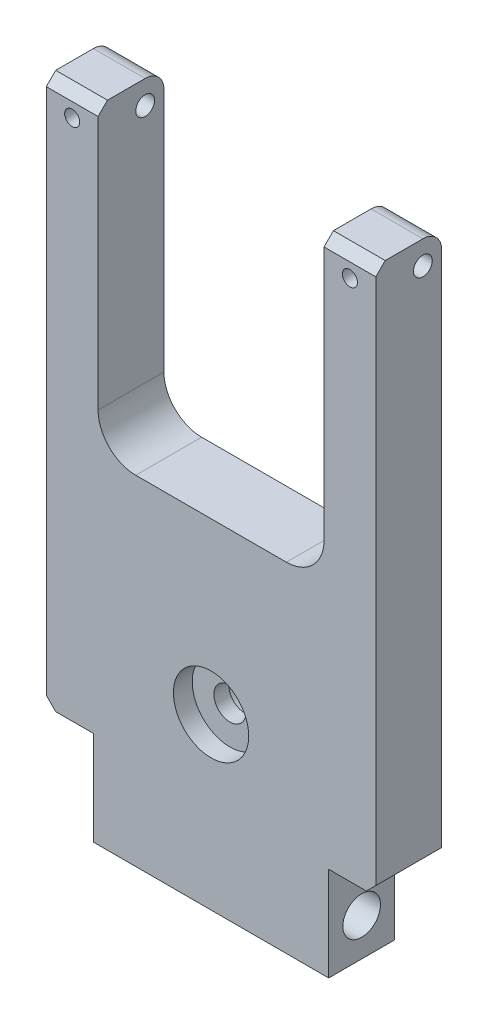
SolidWorks part; units mm, degrees
material "S45C"
ref_plane "Front Plane" through (0, 0, 0) normal (0, 0, 1) x (1, 0, 0)
ref_plane "Top Plane" through (0, 0, 0) normal (0, 1, 0) x (1, 0, 0)
ref_plane "Right Plane" through (0, 0, 0) normal (1, 0, 0) x (0, 0, -1)
sketch "Sketch1" plane through (0, 0, 0) normal (0, 0, 1) x (1, 0, 0)
  line L0 (17.5, 0) -> (-17.5, 0)
  line L1 (-17.5, 0) -> (-17.5, 68)
  line L2 (-17.5, 68) -> (-12, 68)
  line L3 (-12, 68) -> (-12, 36)
  line L4 (-12, 36) -> (12, 36)
  line L5 (0, 0) -> (0, 36) construction
  line L6 (12, 68) -> (12, 36)
  line L7 (17.5, 68) -> (12, 68)
  line L8 (17.5, 0) -> (17.5, 68)
  dimension "D1" = 35
  dimension "D2" = 24
  dimension "D3" = 32
  dimension "D4" = 68
extrude "Boss-Extrude1" add sketch "Sketch1" along normal blind 7
sketch "Sketch2" plane through (17.5, 0, 0) normal (1, 0, 0) x (0, 0, -1)
  line L0 (0, 0) -> (0, 68) construction
  line L1 (-7, 68) -> (0, 68) construction
  circle A0 centre (-2, 65.5) radius 1
  dimension "D1" = 2
  dimension "D2" = 2
  dimension "D3" = 2.5
extrude "Cut-Extrude1" cut sketch "Sketch2" against normal through all
sketch "Sketch3" plane through (0, 0, 7) normal (0, 0, 1) x (1, 0, 0)
  line L0 (0, 0) -> (0, 36) construction
  line L1 (-17.5, 0) -> (-12.5, 0)
  line L2 (-17.5, 0) -> (-17.5, 10)
  line L3 (-17.5, 10) -> (-12.5, 10)
  line L4 (-12.5, 0) -> (-12.5, 10)
  line L5 (12, 36) -> (-12, 36) construction
  line L6 (12.5, 0) -> (12.5, 10)
  line L7 (17.5, 10) -> (12.5, 10)
  line L8 (17.5, 0) -> (17.5, 10)
  line L9 (17.5, 0) -> (12.5, 0)
  dimension "D1" = 25
  dimension "D2" = 10
extrude "Cut-Extrude2" cut sketch "Sketch3" against normal through all
sketch "Sketch4" plane through (12.5, 0, 0) normal (1, 0, 0) x (0, 0, -1)
  line L0 (0, 10) -> (0, 0) construction
  line L1 (0, 0) -> (-7, 0) construction
  circle A0 centre (-3.5, 4) radius 2
  dimension "D1" = 4
  dimension "D2" = 3.5
  dimension "D3" = 4
extrude "Cut-Extrude3" cut sketch "Sketch4" against normal through all
hole_wizard "M3 Tapped Hole1" positions "Sketch6" profile "Sketch7" tap size "M3" standard "GB"
sketch "Sketch6" plane through (0, 0, 0) normal (0, -1, 0) x (1, 0, 0)
  line L0 (-7.5, 3.5) -> (7.5, 3.5) construction
  line L3 (0, 3.5) -> (0, 0) construction
  point P0 (7.5, 3.5)
  point P1 (-7.5, 3.5)
  dimension "D1" = 3.5
  dimension "D2" = 15
sketch "Sketch7" plane through (7.5, 0, 3.5) normal (1, 0, 0) x (0, 0, -1)
  line L0 (0, 0) -> (0, 2)
  line L1 (0, 2) -> (1.25, 2)
  line L2 (1.25, 2) -> (1.25, 0)
  line L5 (1.25, 0) -> (0, 0)
  line L11 (0, -6.35) -> (0, 107.95) construction
  dimension "通孔螺纹孔钻头直径" = 2.5
  dimension "通孔螺纹孔钻头深度" = 2
cosmetic thread "Cosmetic Thread 1" parameters "D2"=3
cosmetic thread "Cosmetic Thread 2" parameters "D2"=3
fillet "Fillet1" radius 4 2 edges at (12, 36, 3.5) (-12, 36, 3.5)
chamfer "Chamfer1" distance 1 angle 45 4 edges at (14.75, 68, 7) (-14.75, 68, 7) (-17.5, 10, 3.5) (17.5, 10, 3.5)
sketch "Sketch8" plane through (0, 0, 7) normal (0, 0, 1) x (1, 0, 0)
  line L0 (-12.5, 0) -> (12.5, 0) construction
  circle A0 centre (0, 18) radius 4
  dimension "D2" = 8
  dimension "D1" = 18
extrude "Cut-Extrude4" cut sketch "Sketch8" against normal blind 2
fillet "Fillet2" radius 2 2 edges at (-14.75, 68, 0) (14.75, 68, 0)
hole_wizard "M2 Tapped Hole1" positions "Sketch10" profile "Sketch9" tap size "M2" standard "GB"
sketch "Sketch10" plane through (0, 0, 7) normal (0, 0, 1) x (1, 0, 0)
  line L0 (12, 68) -> (17.5, 68) construction
  line L1 (-12, 40) -> (-12, 67) construction
  line L2 (12, 67) -> (12, 40) construction
  point P0 (-14.75, 65.5)
  point P1 (14.75, 65.5)
  dimension "D1" = 2.5
  dimension "D2" = 2.75
  dimension "D3" = 2.75
sketch "Sketch9" plane through (-14.75, 65.5, 7) normal (1, 0, 0) x (0, -1, 0)
  line L0 (0, 0) -> (0, 5.6807)
  line L1 (0, 5.6807) -> (0.8, 5.2)
  line L2 (0.8, 5.2) -> (0.8, 0)
  line L5 (0.8, 0) -> (0, 0)
  line L10 (0, 5.6807) -> (-0.8, 5.2) construction
  line L11 (0, -6.35) -> (0, 107.95) construction
  dimension "螺纹孔钻头直径" = 1.6
  dimension "螺纹孔钻头深度" = 5.2
  dimension "导头角度" = 118
cosmetic thread "Cosmetic Thread 3" parameters "D1"=4, "D2"=2
cosmetic thread "Cosmetic Thread 4" parameters "D1"=4, "D2"=2
hole_wizard "CBORE for M3 Hex Socket Head Cap Screw1" positions "Sketch12" profile "Sketch11" counterbore size "M3" standard "Iso" end condition through all
sketch "Sketch12" plane through (0, 0, 0) normal (0, 0, -1) x (-1, 0, 0)
  line L0 (0, 0) -> (0, 36) construction
  line L1 (-8, 36) -> (8, 36) construction
  line L3 (12.5, 0) -> (-12.5, 0) construction
  point P0 (0, 18)
  dimension "D1" = 18
sketch "Sketch11" plane through (0, 18, 0) normal (1, 0, 0) x (0, 1, 0)
  line L0 (0, 0) -> (0, 7)
  line L1 (0, 7) -> (1.7, 7)
  line L3 (1.7, 7) -> (1.7, 3.4)
  line L4 (1.7, 3.4) -> (3.25, 3.4)
  line L5 (3.25, 3.4) -> (3.25, 0)
  line L7 (3.25, 0) -> (0, 0)
  line L11 (0, -6.35) -> (0, 107.95) construction
  dimension "通孔孔直径" = 3.4
  dimension "通孔孔深度" = 7
  dimension "柱形沉头孔直径" = 6.5
  dimension "柱形沉头孔深度" = 3.4
